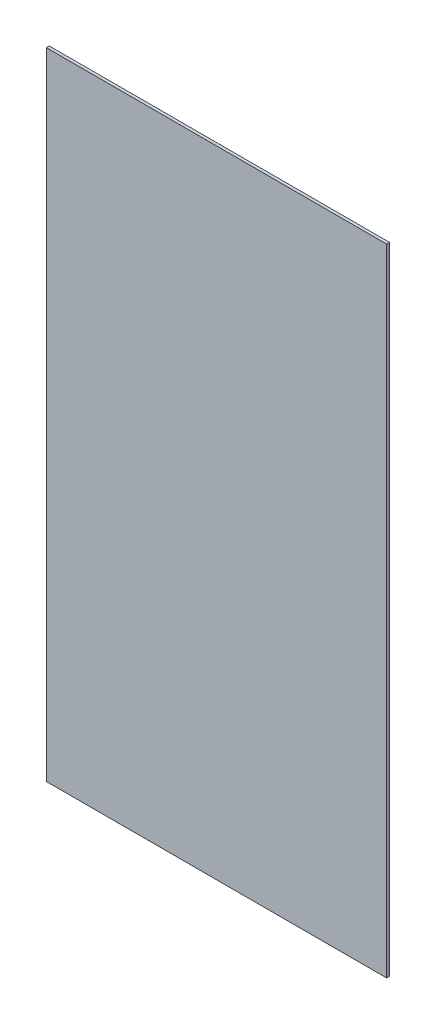
from build123d import *

# Parameters (mm, degrees)
SKETCH_1_W      = 584
SKETCH_1_H      = 1091
EXTRUDE_1_DEPTH = 5


with BuildPart() as part:
    # 草图1 → 凸台-拉伸1 (new body)
    with BuildSketch(Plane.XY):
        Rectangle(SKETCH_1_W, SKETCH_1_H)
    extrude(amount=EXTRUDE_1_DEPTH)


solid = part.part
